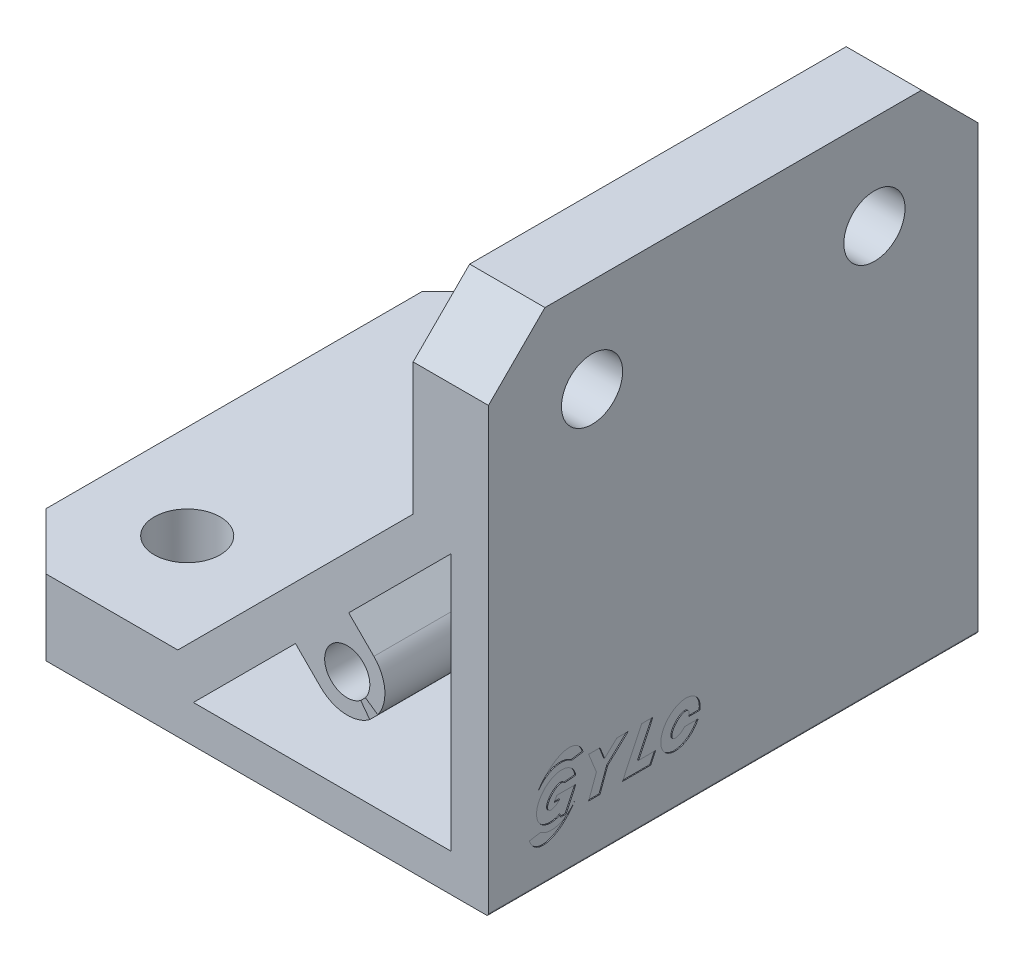
SolidWorks part; units mm, degrees
ref_plane "前视" through (0, 0, 0) normal (0, 0, 1) x (1, 0, 0)
ref_plane "上视" through (0, 0, 0) normal (0, 1, 0) x (1, 0, 0)
ref_plane "右视" through (0, 0, 0) normal (1, 0, 0) x (0, 0, -1)
sketch "Model" plane through (0, 0, 0) normal (0, 0, 1) x (1, 0, 0)
  line L0 (352.7976, 146.5885) -> (380.1407, 146.5885)
  line L1 (366.3123, 154.7601) -> (363.6407, 157.4317)
  line L2 (380.1407, 146.5885) -> (380.1407, 173.9317)
  line L3 (380.1407, 173.9317) -> (369.2976, 163.0885)
  line L4 (371.9691, 160.417) -> (369.2976, 163.0885)
  line L5 (376.1407, 195.5885) -> (384.1407, 195.5885)
  line L6 (331.1407, 150.5885) -> (331.1407, 142.5885)
  line L7 (363.6407, 157.4317) -> (352.7976, 146.5885)
  line L8 (370.5741, 155.6636) -> (371.5298, 154.3804)
  line L9 (335.1407, 146.5885) -> (380.1407, 146.5885) construction
  line L10 (380.1407, 146.5885) -> (380.1407, 191.5885) construction
  line L11 (380.1407, 173.9317) -> (352.7976, 146.5885) construction
  line L12 (376.1407, 175.5885) -> (351.1407, 150.5885)
  line L13 (371.0722, 156.164) -> (372.3859, 155.2501)
  line L22 (351.1407, 150.5885) -> (331.1407, 150.5885)
  line L24 (331.1407, 142.5885) -> (383.9037, 142.5885)
  line L25 (384.1407, 142.8255) -> (384.1407, 195.5885)
  line L27 (376.1407, 195.5885) -> (376.1407, 175.5885)
  line L28 (352.7976, 146.5885) -> (335.1407, 146.5885) construction
  line L29 (380.1407, 191.5885) -> (380.1407, 173.9317) construction
  line L30 (335.1407, 146.5885) -> (335.1407, 146.5885) construction
  line L31 (380.1407, 191.5885) -> (380.1407, 191.5885) construction
  arc A0 (371.0722, 156.164) -> (370.5741, 155.6636) centre (369.1407, 157.5885) ccw
  arc A1 (366.3123, 154.7601) -> (371.5298, 154.3804) centre (369.1407, 157.5885) ccw
  arc A2 (372.3859, 155.2501) -> (371.9691, 160.417) centre (369.1407, 157.5885) ccw
  arc A15 (383.9037, 142.5885) -> (384.1407, 142.8255) centre (383.9037, 142.8255) ccw
  arc A16 (380.1407, 146.5885) -> (380.1407, 146.5885) centre (380.1407, 146.5885) ccw construction
  dimension "D8" = 4.8
  dimension "D10" = 8
  dimension "D1" = 53
  dimension "D2" = 53
  dimension "D3" = 8
  dimension "D4" = 8
  dimension "D5" = 4
  dimension "D6" = 15
  dimension "D7" = 15
  dimension "D9" = 20
  dimension "D11" = 20
extrude "凸台-拉伸1" add sketch "Model" along normal blind 52
sketch "草图1" plane through (0, 142.5885, 0) normal (0, -1, 0) x (-1, 0, 0)
  line L0 (-331.1407, 0) -> (-383.9037, 0) construction
  line L1 (-331.1407, -52) -> (-331.1407, 0) construction
  circle A0 centre (-341.1407, -11) radius 3.5
  circle A3 centre (-341.1407, -41) radius 3.5
  dimension "D1" = 11
  dimension "D2" = 10
  dimension "D3" = 7
  dimension "D6" = 30
extrude "切除-拉伸1" cut sketch "草图1" against normal blind 10
sketch "草图3" plane through (384.1407, 0, 0) normal (1, 0, 0) x (0, 0, -1)
  line L2 (-52, 142.8255) -> (-52, 195.5885) construction
  line L4 (-52, 195.5885) -> (0, 195.5885) construction
  circle A1 centre (-41, 185.5885) radius 3.25
  circle A2 centre (-11, 185.5885) radius 3.25
  dimension "D1" = 11
  dimension "D2" = 6.5
  dimension "D3" = 10
  dimension "D5" = 30
extrude "切除-拉伸2" cut sketch "草图3" against normal blind 10
sketch "草图4" plane through (384.1407, 0, 0) normal (1, 0, 0) x (0, 0, -1)
  line L0 (-52, 142.8255) -> (-50.8, 142.8255) construction
  line L1 (-50.8, 142.8255) -> (-49.6, 142.8255) construction
  line L2 (-49.6, 142.8255) -> (-48.4, 142.8255) construction
  line L3 (-48.4, 142.8255) -> (-47.2, 142.8255) construction
  line L4 (-47.2, 142.8255) -> (-46, 142.8255) construction
  line L5 (-46, 142.8255) -> (-44.8, 142.8255) construction
  line L6 (-44.8, 142.8255) -> (-43.6, 142.8255) construction
  line L7 (-52, 142.8255) -> (-52, 141.6255) construction
  line L8 (-52, 141.6255) -> (-52, 140.4255) construction
  line L9 (-52, 140.4255) -> (-52, 139.2255) construction
  line L10 (-52, 142.2255) -> (-49.6, 142.2255) construction
  line L11 (-52, 141.6255) -> (-48.4, 141.6255) construction
  line L12 (-52, 140.4255) -> (-46, 140.4255) construction
  line L13 (-52, 141.0255) -> (-47.2, 141.0255) construction
  line L14 (-52, 139.8255) -> (-44.8, 139.8255) construction
  line L15 (-52, 139.2255) -> (-43.6, 139.2255) construction
  line L16 (-31.6, 150.0255) -> (-29.9817, 151.7979) construction
  line L17 (-31.6, 150.0255) -> (-44.8, 150.0255) construction
  line L18 (-31.1569, 149.6209) -> (-29.7349, 149.6209)
  line L19 (-31.1569, 149.6209) -> (-31.6, 150.0255) construction
  line L20 (-31.6, 150.0255) -> (-32.9293, 151.2392) construction
  line L21 (-31.6, 150.0255) -> (-32.4091, 149.1393) construction
  line L22 (-49.6, 142.8255) -> (-49.6, 142.2255) construction
  line L23 (-47.2, 142.8255) -> (-47.2, 141.0255) construction
  line L24 (-44.8, 150.0255) -> (-43.1817, 151.7979) construction
  line L25 (-43.9256, 150.8267) -> (-42.7301, 150.9313)
  line L26 (-44.3569, 149.6209) -> (-44.8, 150.0255) construction
  line L27 (-44.8, 150.0255) -> (-46.1293, 151.2392) construction
  line L28 (-44.8, 150.0255) -> (-45.6091, 149.1393) construction
  line L29 (-30.7272, 150.3243) -> (-29.5272, 150.3243)
  line L30 (-44.3569, 148.1361) -> (-44.3569, 147.8774)
  line L31 (-44.7414, 150.0897) -> (-42.7134, 150.0897)
  line L32 (-42.7134, 150.0897) -> (-43.7569, 147.8774)
  line L33 (-43.7569, 147.8774) -> (-44.3569, 147.8774)
  line L34 (-44.7414, 150.0897) -> (-45.0175, 149.557)
  line L35 (-45.0175, 149.557) -> (-44.4175, 149.557)
  line L36 (-43.6, 142.8255) -> (-42.4, 142.8255) construction
  line L37 (-42.4, 142.8255) -> (-41.2, 142.8255) construction
  line L38 (-41.2, 142.8255) -> (-40, 142.8255) construction
  line L39 (-52, 139.2255) -> (-52, 138.0255) construction
  line L40 (-52, 138.0255) -> (-38.8, 138.0255) construction
  line L41 (-41.3569, 147.8774) -> (-40.1569, 147.8774)
  line L42 (-41.3569, 147.8774) -> (-40.5361, 150.1327)
  line L43 (-39.3361, 150.1327) -> (-37.1569, 152.1736)
  line L44 (-37.1569, 152.1736) -> (-38.3569, 152.1736)
  line L45 (-38.3569, 152.1736) -> (-39.6644, 150.949)
  line L46 (-39.6644, 150.949) -> (-40.1569, 152.1736)
  line L47 (-40.1569, 152.1736) -> (-41.3569, 152.1736)
  line L48 (-41.3569, 152.1736) -> (-40.5361, 150.1327)
  line L49 (-39.3361, 150.1327) -> (-40.1569, 147.8774)
  line L50 (-41.3569, 147.8774) -> (-43.7569, 147.8774) construction
  line L51 (-35.7304, 152.1736) -> (-37.7569, 147.8774)
  line L52 (-52, 138.6255) -> (-40, 138.6255) construction
  line L53 (-40, 142.8255) -> (-40, 138.6255) construction
  line L54 (-37.7569, 147.8774) -> (-34.7569, 147.8774)
  line L55 (-34.7569, 147.8774) -> (-34.245, 148.9627)
  line L56 (-34.245, 148.9627) -> (-36.045, 148.9627)
  line L57 (-36.045, 148.9627) -> (-34.5304, 152.1736)
  line L58 (-34.5304, 152.1736) -> (-35.7304, 152.1736)
  line L59 (-37.7569, 147.8774) -> (-40.1569, 147.8774) construction
  line L60 (-44.8, 142.8255) -> (-44.8, 139.8255) construction
  line L61 (-38.3569, 152.1736) -> (-40.1569, 152.1736) construction
  line L62 (-43.1307, 152.5159) -> (-41.9452, 152.7016)
  line L63 (-47.6548, 147.3494) -> (-46.4693, 147.5351)
  line L64 (-43.2506, 152.5944) -> (-44.8, 150.0255) construction
  line L65 (-42.7449, 148.786) -> (-44.8, 150.0255) construction
  line L66 (-44.8, 150.0255) -> (-46.9692, 146.429) construction
  line L67 (-42.4, 142.8255) -> (-42.4, 138.6255) construction
  line L68 (-46, 142.8255) -> (-46, 140.4255) construction
  line L69 (-40, 142.8255) -> (-38.8, 142.8255) construction
  line L70 (-52, 142.8255) -> (-52, 150.0255) construction
  line L71 (-52, 150.0255) -> (-44.8, 150.0255) construction
  line L72 (-52, 150.0255) -> (-52, 157.2255) construction
  ellipse E0 centre (-31.6, 150.0255) end of major axis (-32.4091, 149.1393) minor radius 0.6 (-30.7272, 150.3243) -> (-31.1569, 149.6209) ccw
  ellipse E1 centre (-31.6, 150.0255) end of major axis (-33.2183, 148.2531) minor radius 1.8 (-29.5272, 150.3243) -> (-29.7349, 149.6209) ccw
  ellipse E2 centre (-44.8, 150.0255) end of major axis (-45.6091, 149.1393) minor radius 0.6 (-43.9256, 150.8267) -> (-44.4175, 149.557) ccw
  ellipse E3 centre (-44.8, 150.0255) end of major axis (-46.4183, 148.2531) minor radius 1.8 (-42.7301, 150.9313) -> (-44.3569, 148.1361) ccw
  ellipse E4 centre (-44.8, 150.0255) end of major axis (-46.9692, 146.429) minor radius 2.4 (-41.9452, 152.7016) -> (-46.8551, 151.265) ccw
  ellipse E5 centre (-44.8, 150.0255) end of major axis (-43.2506, 152.5944) minor radius 2.4 (-43.1307, 152.5159) -> (-46.8551, 151.265) ccw
  ellipse E6 centre (-44.8, 150.0255) end of major axis (-42.6308, 153.622) minor radius 2.4 (-47.6548, 147.3494) -> (-42.7449, 148.786) ccw
  ellipse E7 centre (-44.8, 150.0255) end of major axis (-43.2506, 152.5944) minor radius 2.4 (-46.4693, 147.5351) -> (-42.7449, 148.786) ccw
  dimension "D1" = 1.2
  dimension "D2" = 70
  dimension "D3" = 47.602
  dimension "D4" = 11.302
  dimension "D5" = 50
  dimension "D6" = 5
  dimension "D7" = 15
extrude "切除-拉伸3" cut sketch "草图4" against normal blind 0.1
chamfer "倒角2" distance 6 angle 45 4 edges at (380.1407, 195.5885, 52) (331.1407, 146.5885, 52) (331.1407, 146.5885, 0) (380.1407, 195.5885, 0)
